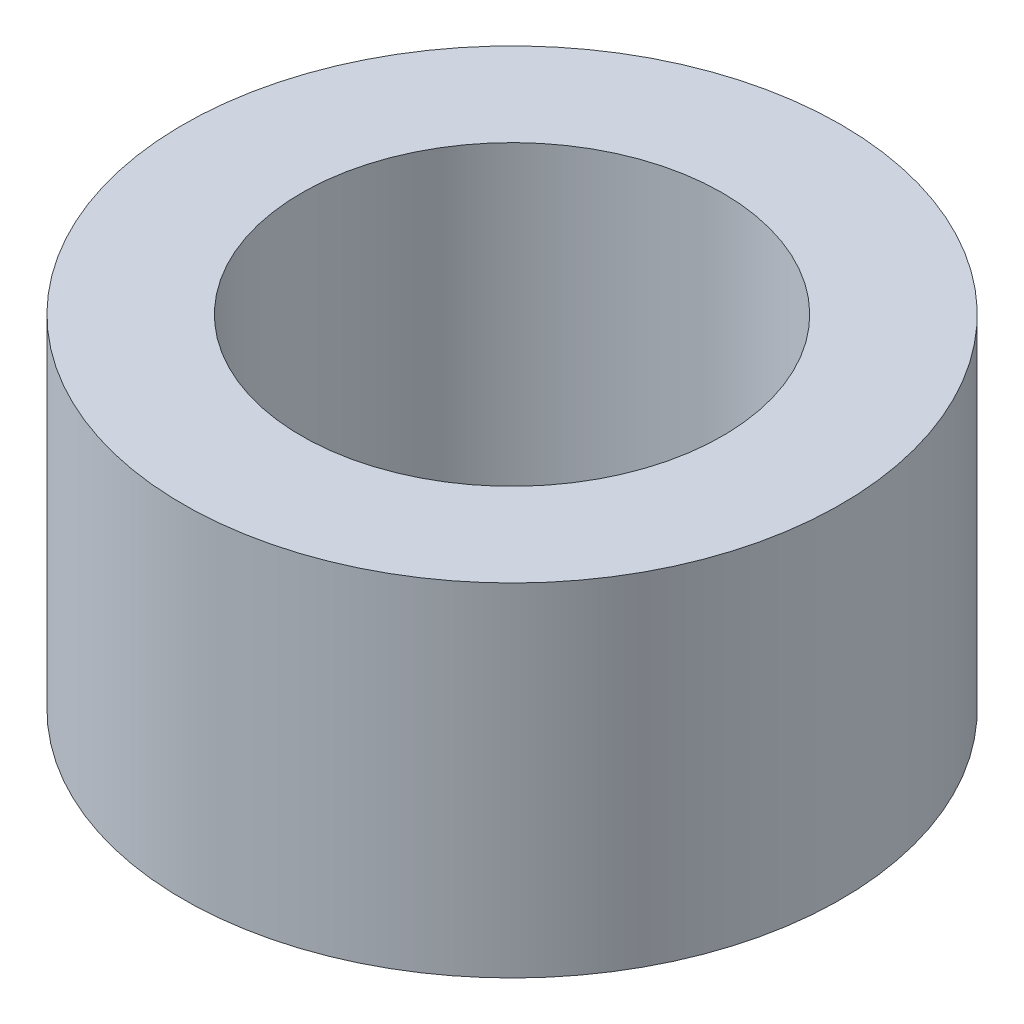
SolidWorks part; units mm, degrees
material "普通碳钢"
ref_plane "前视" through (0, 0, 0) normal (0, 0, 1) x (1, 0, 0)
ref_plane "上视" through (0, 0, 0) normal (0, 1, 0) x (1, 0, 0)
ref_plane "右视" through (0, 0, 0) normal (1, 0, 0) x (0, 0, -1)
sketch "草图1" plane through (0, 0, 0) normal (0, 1, 0) x (1, 0, 0)
  circle A0 centre (0, 0) radius 8
  circle A1 centre (0, 0) radius 12.5
  dimension "D1" = 16
  dimension "D2" = 25
extrude "凸台-拉伸1" add sketch "草图1" along normal blind 13
